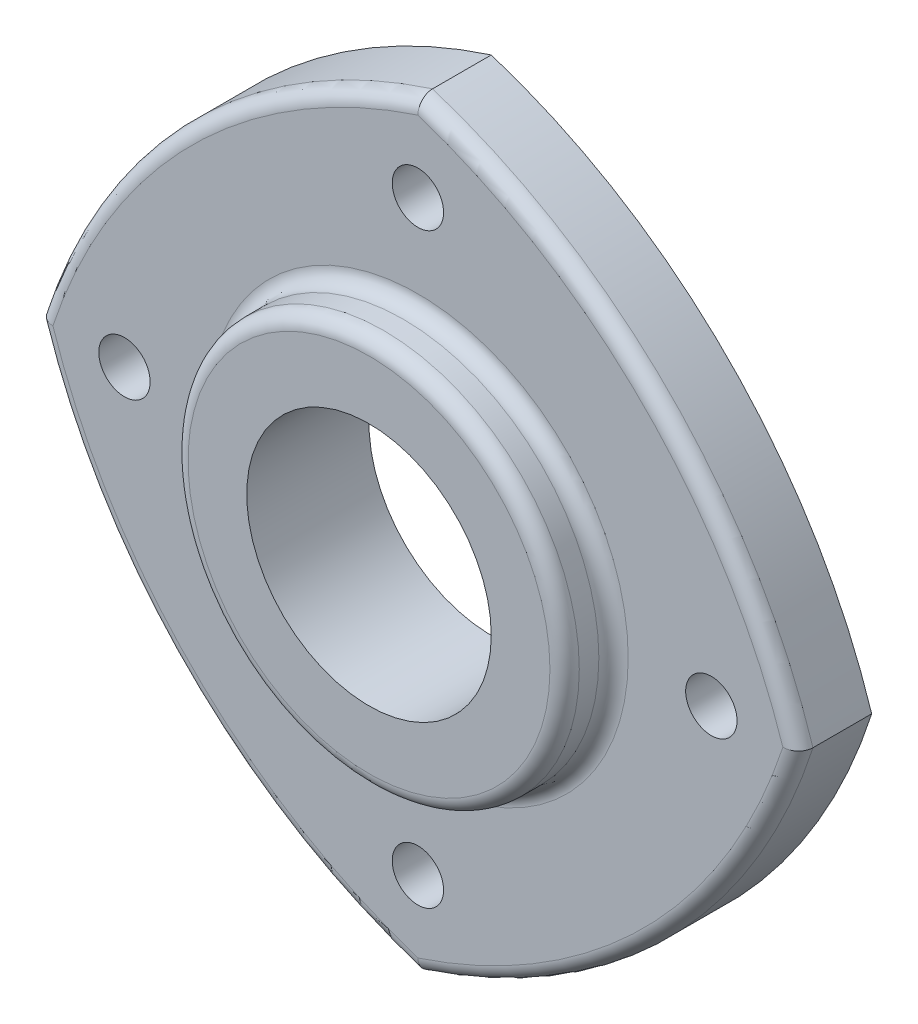
from build123d import *

# Parameters (mm, degrees)
SKETCH_1_R          = 5.25
EXTRUDE_1_DEPTH     = 15
SKETCH_2_R          = 40
EXTRUDE_2_DEPTH     = 10
SKETCH_3_R          = 25
CUT_EXTRUDE_1_DEPTH = 113.805141727
FILLET_1_R          = 3


with BuildPart() as part:
    # 草图1 → 凸台-拉伸1 (new body)
    with BuildSketch(Plane.XY):
        with BuildLine():
            ThreePointArc((0, 77.781745931), (48.328171063, 48.328171063), (77.781745931, 0))
            ThreePointArc((77.781745931, 0), (48.328171063, -48.328171063), (0, -77.781745931))
            ThreePointArc((0, -77.781745931), (-48.328171063, -48.328171063), (-77.781745931, 0))
            ThreePointArc((-77.781745931, 0), (-48.328171063, 48.328171063), (0, 77.781745931))
        make_face()
        with Locations((0, 60)):
            Circle(SKETCH_1_R, mode=Mode.SUBTRACT)
        with Locations((60, 0)):
            Circle(SKETCH_1_R, mode=Mode.SUBTRACT)
        with Locations((0, -60)):
            Circle(SKETCH_1_R, mode=Mode.SUBTRACT)
        with Locations((-60, 0)):
            Circle(SKETCH_1_R, mode=Mode.SUBTRACT)
    extrude(amount=EXTRUDE_1_DEPTH)

    # 草图2 → 凸台-拉伸2 (add)
    with BuildSketch(Plane.XY.offset(15)):
        with Locations(Location((0, 0, 0), (0, 0, 180))):
            Circle(SKETCH_2_R)
    extrude(amount=EXTRUDE_2_DEPTH)

    # 草图3 → 切除-拉伸1 (cut, through all)
    with BuildSketch(Plane.XY.offset(25)):
        Circle(SKETCH_3_R)
    extrude(amount=-CUT_EXTRUDE_1_DEPTH, mode=Mode.SUBTRACT)

    # 圆角1
    fillet_1_edges = [part.edges().sort_by_distance(p)[0] for p in [
        (48.328171063, -48.328171063, 15),
        (48.328171063, 48.328171063, 15),
        (40, 0, 15),
        (40, 0, 25),
        (-48.328171063, 48.328171063, 15),
        (-48.328171063, -48.328171063, 15),
    ]]
    fillet(fillet_1_edges, radius=FILLET_1_R)


solid = part.part
